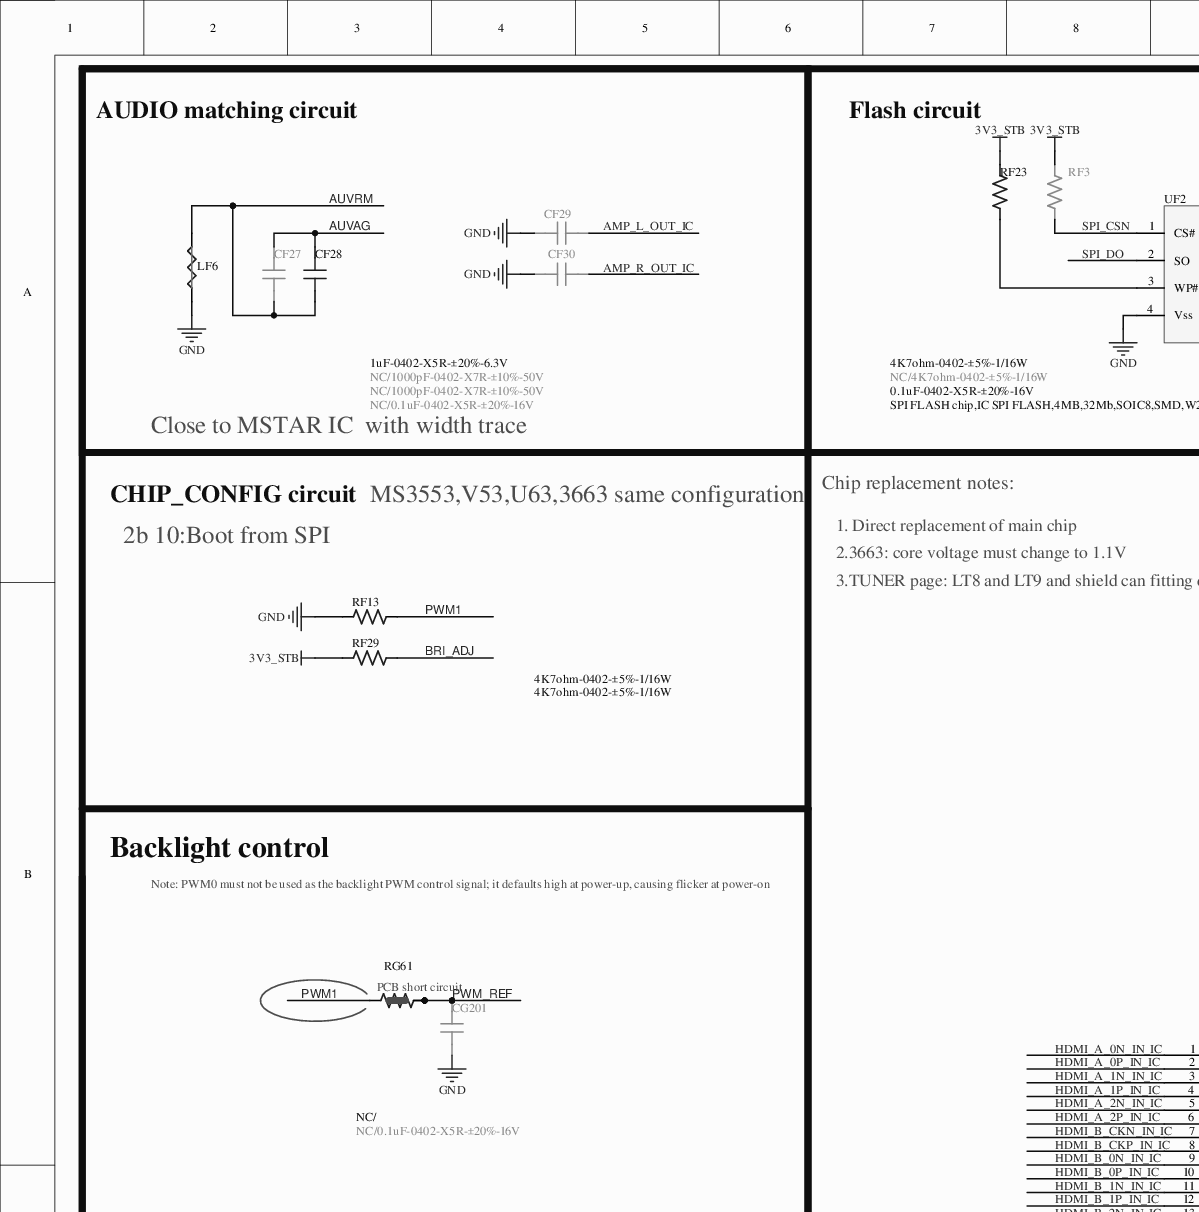
[diagram p0: MISC86372-9.SchDoc, top left]
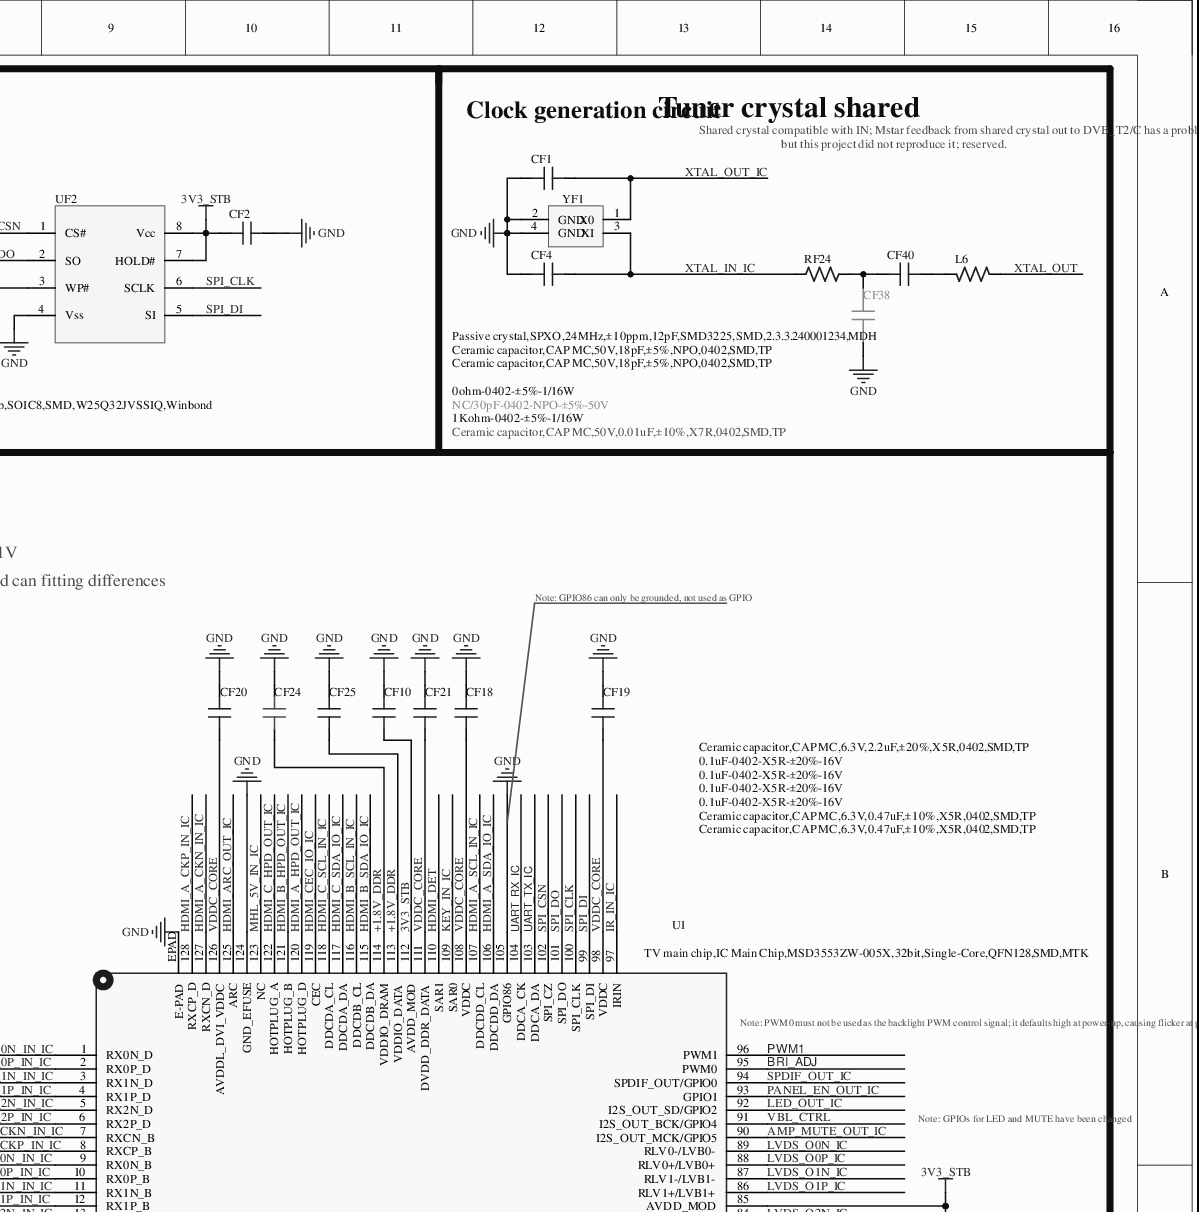
[diagram p1: MISC86372-9.SchDoc, top right]
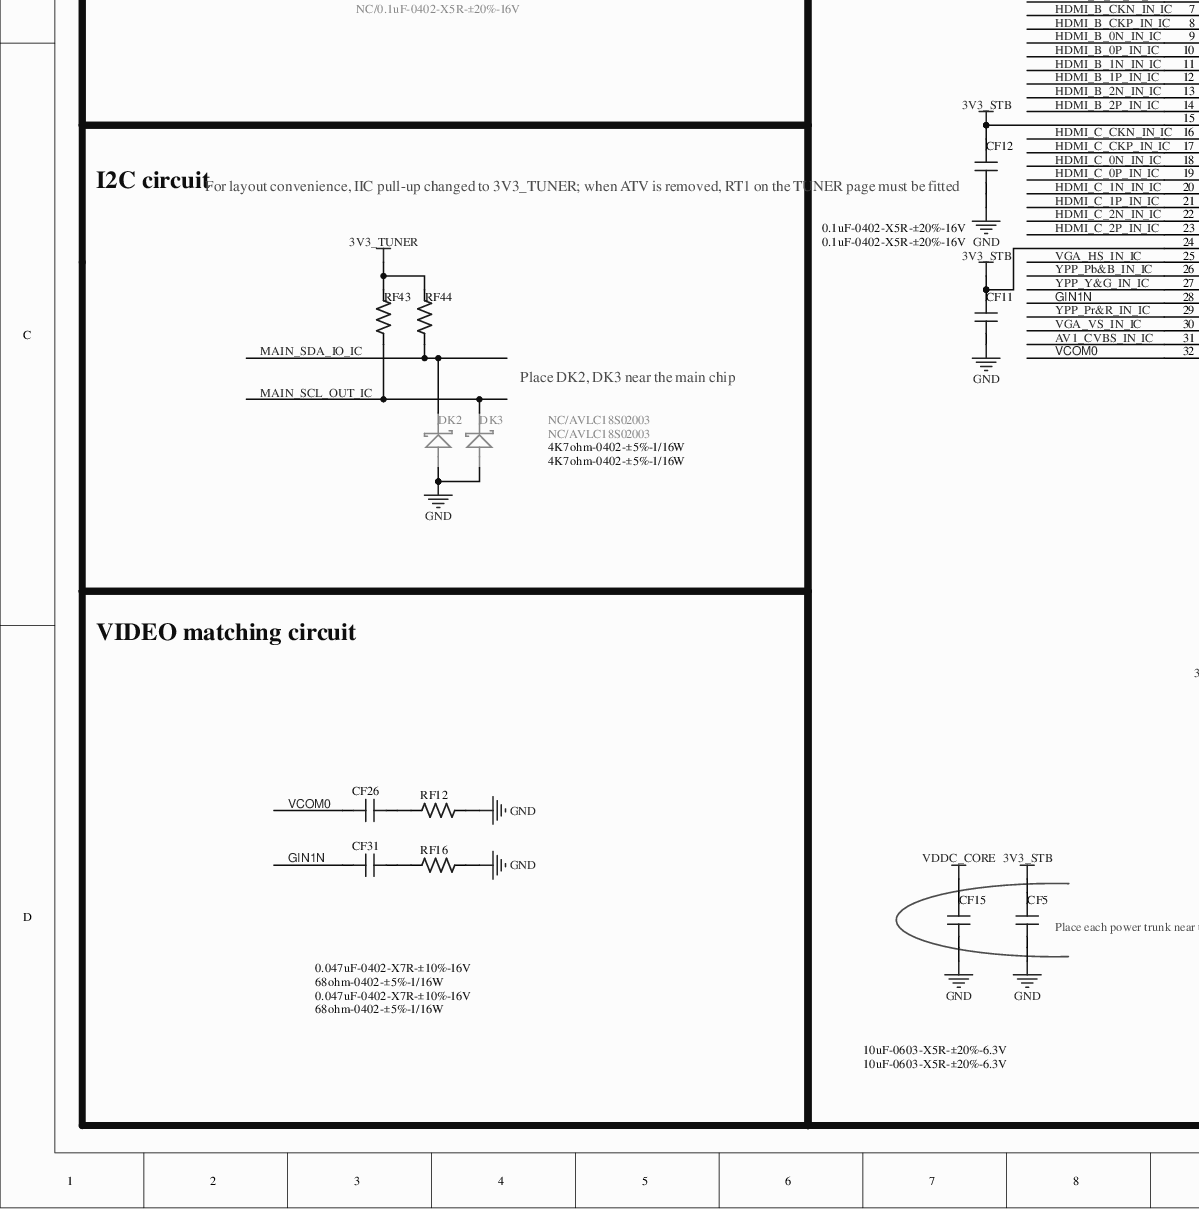
[diagram p2: MISC86372-9.SchDoc, bottom left]
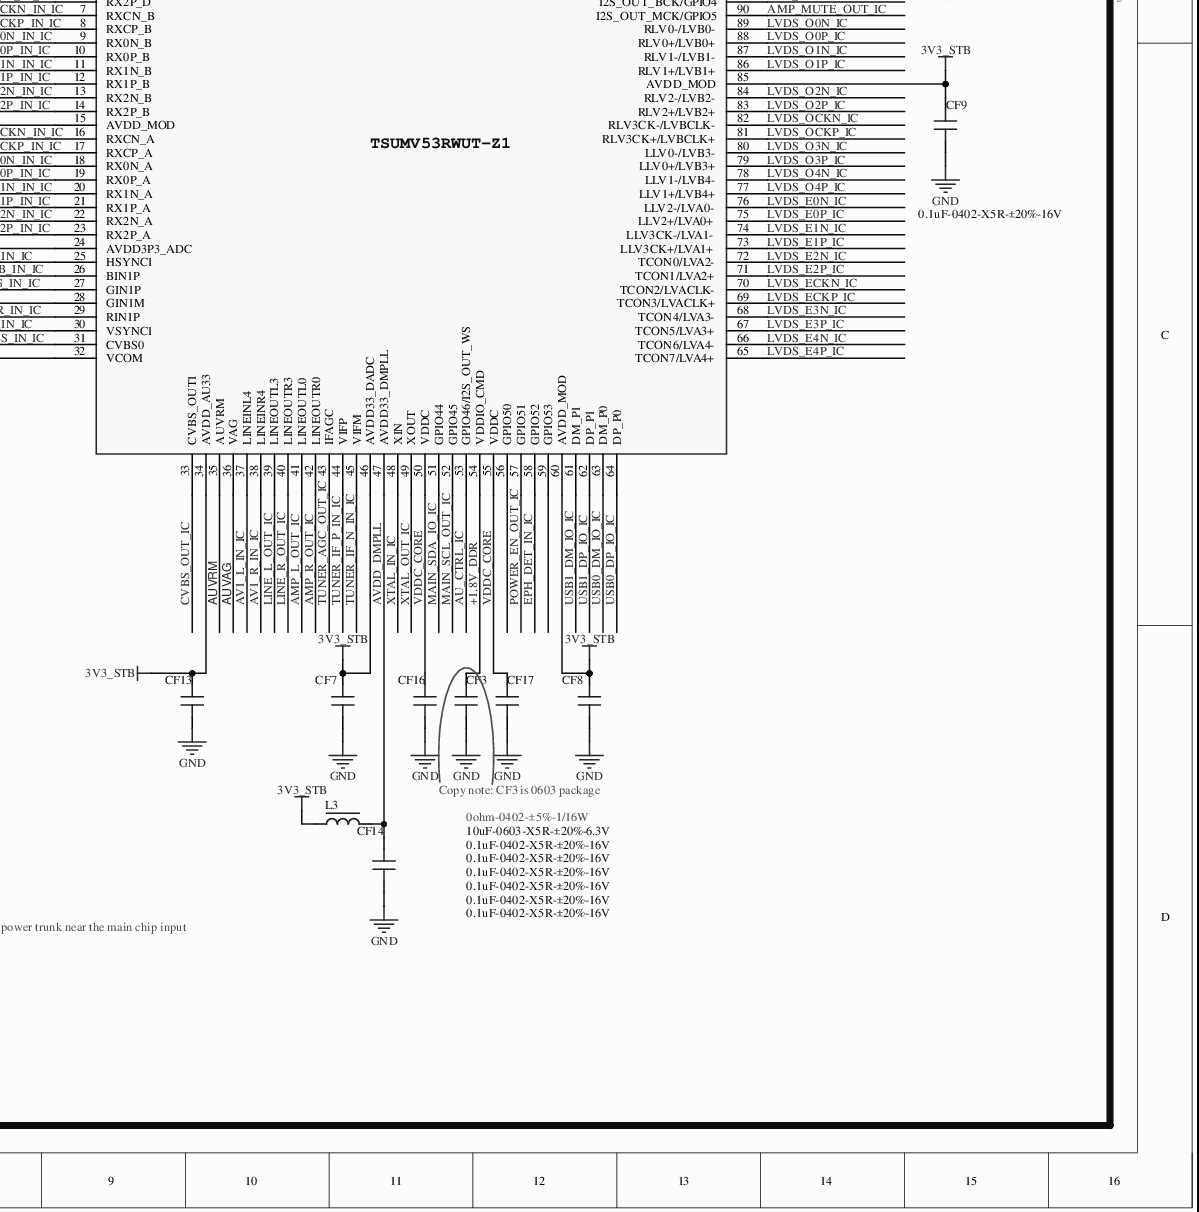
[diagram p3: MISC86372-9.SchDoc, bottom right]
# Altium project MISC86372-32.PrjPCB (part 3 of 8)

## Sheet MISC86372-9.SchDoc
size 426 x 431 mm

### Parts
CF1  Ceramic capacitor,CAP MC,50V,18pF,±5%,NPO,0402,SMD,TP  [C0402]
CF2  0.1uF-0402-X5R-±20%-16V  [C0402]
CF3  10uF-0603-X5R-±20%-6.3V  [C0603]
CF4  Ceramic capacitor,CAP MC,50V,18pF,±5%,NPO,0402,SMD,TP  [C0402]
CF5  10uF-0603-X5R-±20%-6.3V  [C0603]
CF7  0.1uF-0402-X5R-±20%-16V  [C0402]
CF8  0.1uF-0402-X5R-±20%-16V  [C0402]
CF9  0.1uF-0402-X5R-±20%-16V  [C0402]
CF10  0.1uF-0402-X5R-±20%-16V  [C0402]
CF11  0.1uF-0402-X5R-±20%-16V  [C0402]
CF12  0.1uF-0402-X5R-±20%-16V  [C0402]
CF13  0.1uF-0402-X5R-±20%-16V  [C0402]
CF14  0.1uF-0402-X5R-±20%-16V  [C0402]
CF15  10uF-0603-X5R-±20%-6.3V  [C0603]
CF16  0.1uF-0402-X5R-±20%-16V  [C0402]
CF17  0.1uF-0402-X5R-±20%-16V  [C0402]
CF18  0.1uF-0402-X5R-±20%-16V  [C0402]
CF19  0.1uF-0402-X5R-±20%-16V  [C0402]
CF20  0.1uF-0402-X5R-±20%-16V  [C0402]
CF21  Ceramic capacitor,CAP MC,6.3V,0.47uF,±10%,X5R,0402,SMD,TP  [C0402]
CF24  Ceramic capacitor,CAP MC,6.3V,2.2uF,±20%,X5R,0402,SMD,TP  [C0402]
CF25  Ceramic capacitor,CAP MC,6.3V,0.47uF,±10%,X5R,0402,SMD,TP  [C0402]
CF26  0.047uF-0402-X7R-±10%-16V  [C0402]
CF27  NC/0.1uF-0402-X5R-±20%-16V  [C0402]
CF28  1uF-0402-X5R-±20%-6.3V  [C0402]
CF29  NC/1000pF-0402-X7R-±10%-50V  [C0402]
CF30  NC/1000pF-0402-X7R-±10%-50V  [C0402]
CF31  0.047uF-0402-X7R-±10%-16V  [C0402]
CF38  NC/30pF-0402-NPO-±5%-50V  [C0402]
CF40  Ceramic capacitor,CAP MC,50V,0.01uF,±10%,X7R,0402,SMD,TP  [C0402]
CG201  NC/0.1uF-0402-X5R-±20%-16V  [C0402]
DK2  NC/AVLC18S02003  [DIODE-S0402]
DK3  NC/AVLC18S02003  [DIODE-S0402]
L3  0ohm-0402-±5%-1/16W  [L0402]
L6  0ohm-0402-±5%-1/16W  [R0402]
LF6  NC/?  [GND]  (value not drawn)
RF3  NC/4K7ohm-0402-±5%-1/16W  [R0402]
RF12  68ohm-0402-±5%-1/16W  [R0402]
RF13  4K7ohm-0402-±5%-1/16W  [R0402]
RF16  68ohm-0402-±5%-1/16W  [R0402]
RF23  4K7ohm-0402-±5%-1/16W  [R0402]
RF24  1Kohm-0402-±5%-1/16W  [R0402]
RF29  4K7ohm-0402-±5%-1/16W  [R0402]
RF43  4K7ohm-0402-±5%-1/16W  [R0402]
RF44  4K7ohm-0402-±5%-1/16W  [R0402]
RG61  NC/  [R0402SC]
U1  TV main chip,IC Main Chip,MSD3553ZW-005X,32bit,Single-Core,QFN128,SMD,MTK  [QFN128/0.35-1-9]
UF2  SPI FLASH chip,IC SPI FLASH,4MB,32Mb,SOIC8,SMD,W25Q32JVSSIQ,Winbond  [SOIC8]
YF1  Passive crystal,SPXO,24MHz,±10ppm,12pF,SMD3225,SMD,2.3.3.240001234,MDH  [XTAL-S-3]

### Blocks framed on the sheet
Flash circuit: CF2 RF3 RF23 UF2
VIDEO matching circuit: CF26 CF31 RF12 RF16

### Nets
3V3_STB: CF2.2 CF5.2 CF7.2 CF8.2 CF9.2 CF10.2 CF11.1 CF12.2 CF13.2 L3.1 RF3.2 RF23.2 RF29.2 U1.15(AVDD_MOD) U1.24(AVDD3P3_ADC) U1.34(AVDD_AU33) U1.46(AVDD33_DADC) U1.60(AVDD_MOD) U1.85(AVDD_MOD) U1.112(AVDD_MOD) UF2.7(HOLD#) UF2.8(Vcc)
3V3_TUNER: RF43.1 RF44.1
+1.8V_DDR: CF3.2 CF24.1 CF25.1 U1.54(VDDIO_CMD) U1.113(VDDIO_DATA) U1.114(VDDIO_DRAM)
GND: CF1.1 CF2.1 CF3.1 CF4.1 CF5.1 CF7.1 CF8.1 CF9.1 CF10.1 CF11.2 CF12.1 CF13.1 CF14.1 CF15.1 CF16.1 CF17.1 CF18.2 CF19.2 CF20.1 CF21.2 CF24.2 CF25.2 CF29.2 CF30.2 CF38.1 CG201.2 DK2.A DK3.A LF6.JP_2K RF12.2 RF13.2 RF16.2 U1.105(GPIO86) U1.124(GND_EFUSE) U1.EPAD(E-PAD) UF2.4(Vss) YF1.2(GND) YF1.4(GND)
PWM_REF: CG201.1 RG61.2 RG61.3
VDDC_CORE: CF15.2 CF16.2 CF17.2 CF18.1 CF19.1 CF20.2 CF21.1 U1.50(VDDC) U1.55(VDDC) U1.98(VDDC) U1.108(VDDC) U1.111(DVDD_DDR_DATA) U1.126(AVDDL_DVI_VDDC)
AMP_L_OUT_IC: CF29.1 U1.41(LINEOUTL0)
AMP_MUTE_OUT_IC: U1.90(I2S_OUT_MCK/GPIO5)
AMP_R_OUT_IC: CF30.1 U1.42(LINEOUTR0)
AU_CTRL_IC: U1.53(GPIO46/I2S_OUT_WS)
AUVAG: CF27.2 CF28.2 U1.36(VAG)
AUVRM: CF27.1 CF28.1 LF6.JP_1K U1.35(AUVRM)
AV1_CVBS_IN_IC: U1.31(CVBS0)
AV1_L_IN_IC: U1.37(LINEINL4)
AV1_R_IN_IC: U1.38(LINEINR4)
AVDD_DMPLL: CF14.2 L3.2 U1.47(AVDD33_DMPLL)
BRI_ADJ: RF29.1 U1.95(PWM0)
CVBS_OUT_IC: U1.33(CVBS_OUT1)
EPH_DET_IN_IC: U1.58(GPIO52)
GIN1N: CF31.1 U1.28(GIN1M)
HDMI_A_0N_IN_IC: U1.1(RX0N_D)
HDMI_A_0P_IN_IC: U1.2(RX0P_D)
HDMI_A_1N_IN_IC: U1.3(RX1N_D)
HDMI_A_1P_IN_IC: U1.4(RX1P_D)
HDMI_A_2N_IN_IC: U1.5(RX2N_D)
HDMI_A_2P_IN_IC: U1.6(RX2P_D)
HDMI_A_CKN_IN_IC: U1.127(RXCN_D)
HDMI_A_CKP_IN_IC: U1.128(RXCP_D)
HDMI_A_HPD_OUT_IC: U1.120(HOTPLUG_D)
HDMI_A_SCL_IN_IC: U1.107(DDCDD_CL)
HDMI_A_SDA_IO_IC: U1.106(DDCDD_DA)
HDMI_ARC_OUT_IC: U1.125(ARC)
HDMI_B_0N_IN_IC: U1.9(RX0N_B)
HDMI_B_0P_IN_IC: U1.10(RX0P_B)
HDMI_B_1N_IN_IC: U1.11(RX1N_B)
HDMI_B_1P_IN_IC: U1.12(RX1P_B)
HDMI_B_2N_IN_IC: U1.13(RX2N_B)
HDMI_B_2P_IN_IC: U1.14(RX2P_B)
HDMI_B_CKN_IN_IC: U1.7(RXCN_B)
HDMI_B_CKP_IN_IC: U1.8(RXCP_B)
HDMI_B_HPD_OUT_IC: U1.121(HOTPLUG_B)
HDMI_B_SCL_IN_IC: U1.116(DDCDB_CL)
HDMI_B_SDA_IO_IC: U1.115(DDCDB_DA)
HDMI_C_0N_IN_IC: U1.18(RX0N_A)
HDMI_C_0P_IN_IC: U1.19(RX0P_A)
HDMI_C_1N_IN_IC: U1.20(RX1N_A)
HDMI_C_1P_IN_IC: U1.21(RX1P_A)
HDMI_C_2N_IN_IC: U1.22(RX2N_A)
HDMI_C_2P_IN_IC: U1.23(RX2P_A)
HDMI_C_CKN_IN_IC: U1.16(RXCN_A)
HDMI_C_CKP_IN_IC: U1.17(RXCP_A)
HDMI_C_HPD_OUT_IC: U1.122(HOTPLUG_A)
HDMI_C_SCL_IN_IC: U1.118(DDCDA_CL)
HDMI_C_SDA_IO_IC: U1.117(DDCDA_DA)
HDMI_CEC_IO_IC: U1.119(CEC)
HDMI_DET: U1.110(SAR1)
IR_IN_IC: U1.97(IRIN)
KEY_IN_IC: U1.109(SAR0)
LED_OUT_IC: U1.92(I2S_OUT_SD/GPIO2)
LINE_L_OUT_IC: U1.39(LINEOUTL3)
LINE_R_OUT_IC: U1.40(LINEOUTR3)
LVDS_E0N_IC: U1.76(LLV2-/LVA0-)
LVDS_E0P_IC: U1.75(LLV2+/LVA0+)
LVDS_E1N_IC: U1.74(LLV3CK-/LVA1-)
LVDS_E1P_IC: U1.73(LLV3CK+/LVA1+)
LVDS_E2N_IC: U1.72(TCON0/LVA2-)
LVDS_E2P_IC: U1.71(TCON1/LVA2+)
LVDS_E3N_IC: U1.68(TCON4/LVA3-)
LVDS_E3P_IC: U1.67(TCON5/LVA3+)
LVDS_E4N_IC: U1.66(TCON6/LVA4-)
LVDS_E4P_IC: U1.65(TCON7/LVA4+)
LVDS_ECKN_IC: U1.70(TCON2/LVACLK-)
LVDS_ECKP_IC: U1.69(TCON3/LVACLK+)
LVDS_O0N_IC: U1.89(RLV0-/LVB0-)
LVDS_O0P_IC: U1.88(RLV0+/LVB0+)
LVDS_O1N_IC: U1.87(RLV1-/LVB1-)
LVDS_O1P_IC: U1.86(RLV1+/LVB1+)
LVDS_O2N_IC: U1.84(RLV2-/LVB2-)
LVDS_O2P_IC: U1.83(RLV2+/LVB2+)
LVDS_O3N_IC: U1.80(LLV0-/LVB3-)
LVDS_O3P_IC: U1.79(LLV0+/LVB3+)
LVDS_O4N_IC: U1.78(LLV1-/LVB4-)
LVDS_O4P_IC: U1.77(LLV1+/LVB4+)
LVDS_OCKN_IC: U1.82(RLV3CK-/LVBCLK-)
LVDS_OCKP_IC: U1.81(RLV3CK+/LVBCLK+)
MAIN_SCL_OUT_IC: DK3.K RF43.2 U1.52(GPIO45)
MAIN_SDA_IO_IC: DK2.K RF44.2 U1.51(GPIO44)
MHL_5V_IN_IC: U1.123(NC)
PANEL_EN_OUT_IC: U1.93(GPIO1)
POWER_EN_OUT_IC: U1.57(GPIO51)
PWM1: RF13.1 RG61.1 U1.96(PWM1)
SPDIF_OUT_IC: U1.94(SPDIF_OUT/GPIO0)
SPI_CLK: U1.100(SPI_CLK) UF2.6(SCLK)
SPI_CSN: RF3.1 U1.102(SPI_CZ) UF2.1(CS#)
SPI_DI: U1.99(SPI_DI) UF2.5(SI)
SPI_DO: U1.101(SPI_DO) UF2.2(SO)
TUNER_AGC_OUT_IC: U1.43(IFAGC)
TUNER_IF_N_IN_IC: U1.45(VIFM)
TUNER_IF_P_IN_IC: U1.44(VIFP)
UART_RX_IC: U1.104(DDCA_CK)
UART_TX_IC: U1.103(DDCA_DA)
USB0_DM_IO_IC: U1.63(DM_P0)
USB0_DP_IO_IC: U1.64(DP_P0)
USB1_DM_IO_IC: U1.61(DM_P1)
USB1_DP_IO_IC: U1.62(DP_P1)
VBL_CTRL: U1.91(I2S_OUT_BCK/GPIO4)
VCOM0: CF26.1 U1.32(VCOM)
VGA_HS_IN_IC: U1.25(HSYNC1)
VGA_VS_IN_IC: U1.30(VSYNC1)
XTAL_IN_IC: CF4.2 RF24.2 U1.48(XIN) YF1.3(XI)
XTAL_OUT: L6.2
XTAL_OUT_IC: CF1.2 U1.49(XOUT) YF1.1(X0)
YPP_Pb&B_IN_IC: U1.26(BIN1P)
YPP_Pr&R_IN_IC: U1.29(RIN1P)
YPP_Y&G_IN_IC: U1.27(GIN1P)
NetCF26_2: CF26.2 RF12.1
NetCF31_2: CF31.2 RF16.1
NetCF38_2: CF38.2 CF40.2 RF24.1
NetCF40_1: CF40.1 L6.1
NetRF23_1: RF23.1 UF2.3(WP#)

Not connected (* = marked no-connect by the designer): U1 56(GPIO50)* 59(GPIO53)*

### Notes on the sheet
- AUDIO matching circuit
- Clock generation circuit
- Tuner crystal shared
- Shared crystal compatible with IN; Mstar feedback from shared crystal out to DVB_T2/C has a problem,
- but this project did not reproduce it; reserved.
- Close to MSTAR IC  with width trace
- CHIP_CONFIG circuit
- MS3553,V53,U63,3663 same configuration
- Chip replacement notes:
- 2b 10:Boot from SPI
- 1. Direct replacement of main chip
- 2.3663: core voltage must change to 1.1V
- 3.TUNER page: LT8 and LT9 and shield can fitting differences
- Note: GPIO86 can only be grounded, not used as GPIO
- Backlight control
- Note: PWM0 must not be used as the backlight PWM control signal; it defaults high at power-up, causing flicker at power-on
- (near U1) Note: PWM0 must not be used as the backlight PWM control signal; it defaults high at power-up, causing flicker at power-on
- Note: GPIOs for LED and MUTE have been changed
- I2C circuit
- (near CF12) For layout convenience, IIC pull-up changed to 3V3_TUNER; when ATV is removed, RT1 on the TUNER page must be fitted
- Place DK2, DK3 near the main chip
- Copy note: CF3 is 0603 package
- (near CF5) Place each power trunk near the main chip input

### Library data of the parts
CF1 CF4 = 004.003.0000527-D: Ceramic capacitor,CAP MC,50V,18pF,±5%,NPO,0402,SMD,TP-D
CF2 CF7-CF10 CF12-CF14 CF17 CF27 CG201 = 0.1uF-0402-Y5V-+80%-20%-16V-D
CF3 CF5 CF15 = 10uF-0603-X5R-±20%-6.3V-D
CF11 CF16 CF18-CF21 CF25 CF28 = 1uF-0402-X5R-±20%-6.3V-D
CF24 = 004.003.0000100-D: Ceramic capacitor,CAP MC,6.3V,2.2uF,±20%,X5R,0402,SMD,TP-D
CF26 CF31 = 0.047uF-0402-X7R-±10%-16V-D
CF29 CF30 = 1000pF-0402-X7R-±10%-50V-D
CF38 CF40 = 30pF-0402-NPO-±5%-50V-D
DK2 DK3 = AVLC18S02003-D
L3 = FCM1005KF-121T06(120ohm-500mA)-D
L6 = 004.002.0000558-D: Thick-film resistor,RES,1/16W,0ohm,±5%,0402,SMD-D
LF6 = GND: Manufacturer: Panasonic; Part Number: ERJ3GEYJ473V; Right: 20; Bottom: 30; CLASS: Discrete; Comments: Digikey
RF3 RF13 RF23 RF29 RF43 RF44 = 4K7ohm-0402-±5%-1/16W-D
RF12 RF16 = 68ohm-0402-±5%-1/16W-D
RF24 = 1Kohm-0402-±5%-1/16W-D
RG61 = 0ohm-0402-PCB-D
U1 = 004.016.0001146-D: TV main chip,IC Main Chip,TSUMV53RWUT-Z1,32bit,Single-Core,QFN128,SMD,Mstar-D
UF2 = SPI FLASH 芯片,IC SPI FLASH,32Mb,SOIC8,SMD,GD25Q32CSIG,GigaDevice-D
YF1 = 16.000MHz±20PPM-10PF-SMD3225-D: NC: GPS; PCB DECAL: TCXO_3225; Source_Path: EM_66_V2.0_201209181010.DSN; Value: 26M/0.5PPM/1.8V